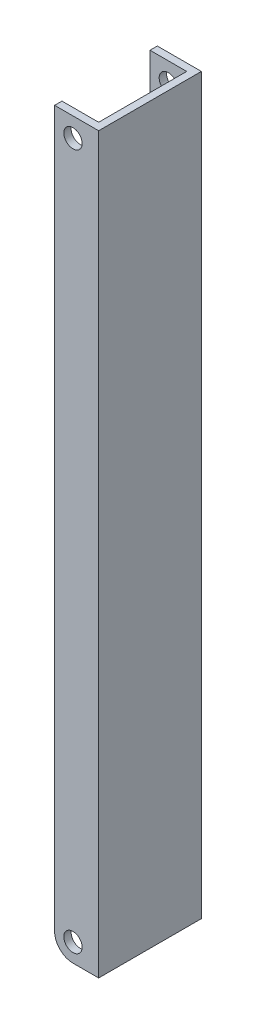
from build123d import *

# Parameters (mm, degrees)
BOSS_EXTRUDE1_DEPTH     = 200
FILLET1_R               = 5
CUT_EXTRUDE1_DEPTH      = 255.356049663
CUT_EXTRUDE1_DEPTH_BACK = 255.356049663
SKETCH3_R               = 2.5
CUT_EXTRUDE2_DEPTH      = 255.356049663
CUT_EXTRUDE2_DEPTH_BACK = 255.356049663
SKETCH9_R               = 2.5


with BuildPart() as part:
    # Sketch2 → Boss-Extrude1 (new body)
    with BuildSketch(Plane(origin=(0, 50, 0), x_dir=(1, 0, 0), z_dir=(0, 1, 0))):
        Polygon((27, 22), (37, 22), (37, -2), (27, -2), (27, -4), (39, -4), (39, 24), (27, 24), align=None)
    extrude(amount=BOSS_EXTRUDE1_DEPTH)

    # Fillet1
    fillet1_edges = [part.edges().sort_by_distance(p)[0] for p in [
        (27, 50, 3),
        (27, 50, -23),
    ]]
    fillet(fillet1_edges, radius=FILLET1_R)

    # Sketch3 → Cut-Extrude1 (cut, two sides: drawn at the far end of the back side and taken through both)
    with BuildSketch(Plane(origin=(0, 0, 2), x_dir=(-1, 0, 0), z_dir=(0, 0, -1)).offset(-CUT_EXTRUDE1_DEPTH_BACK)):
        with Locations((-32, 55)):
            Circle(SKETCH3_R)
    extrude(amount=CUT_EXTRUDE1_DEPTH + CUT_EXTRUDE1_DEPTH_BACK, mode=Mode.SUBTRACT)

    # Sketch9 → Cut-Extrude2 (cut, two sides: drawn at the far end of the back side and taken through both)
    with BuildSketch(Plane(origin=(0, 0, -22), x_dir=(-1, 0, 0), z_dir=(0, 0, -1)).offset(-CUT_EXTRUDE2_DEPTH_BACK)):
        with Locations(Location((-32, 244.730145932, 0), (0, 0, 90))):
            Circle(SKETCH9_R)
    extrude(amount=CUT_EXTRUDE2_DEPTH + CUT_EXTRUDE2_DEPTH_BACK, mode=Mode.SUBTRACT)


solid = part.part
